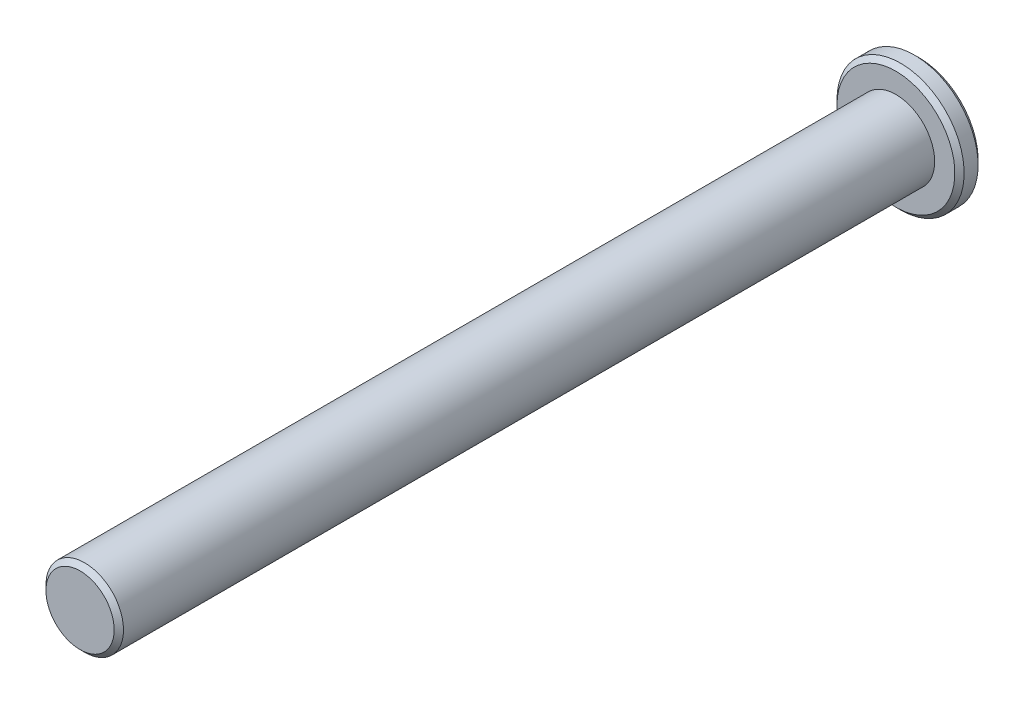
from build123d import *

# Parameters (mm, degrees)
SKETCH1_R           = 25
BOSS_EXTRUDE1_DEPTH = 526
SKETCH2_R           = 41
BOSS_EXTRUDE2_DEPTH = 15
CHAMFER1_SIZE       = 3


with BuildPart() as part:
    # Sketch1 → Boss-Extrude1 (new body)
    with BuildSketch(Plane.XY):
        Circle(SKETCH1_R)
    extrude(amount=BOSS_EXTRUDE1_DEPTH)

    # Sketch2 → Boss-Extrude2 (add)
    with BuildSketch(Plane(origin=(0, 0, 0), x_dir=(-1, 0, 0), z_dir=(0, 0, -1))):
        Circle(SKETCH2_R)
    extrude(amount=BOSS_EXTRUDE2_DEPTH)

    # Chamfer1
    chamfer1_edges = [part.edges().sort_by_distance(p)[0] for p in [
        (-25, 0, 526),
        (41, 0, 0),
        (41, 0, -15),
    ]]
    chamfer(chamfer1_edges, length=CHAMFER1_SIZE)


solid = part.part
